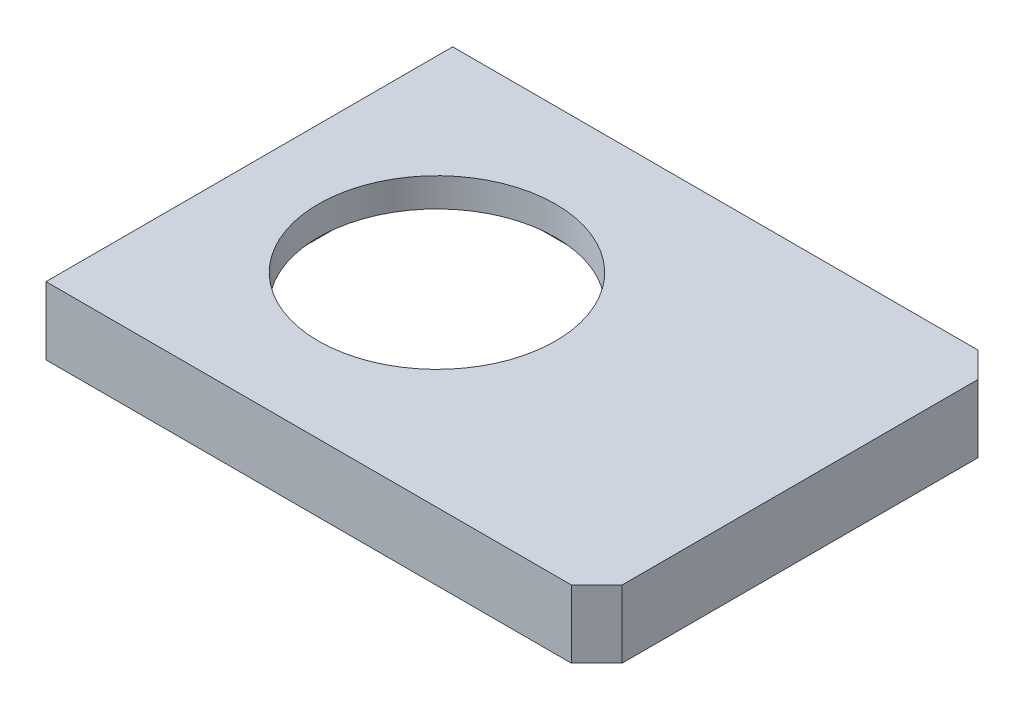
from build123d import *

# Parameters (mm, degrees)
SKETCH_1_W          = 325
SKETCH_1_H          = 240
EXTRUDE_1_DEPTH     = 40
SKETCH_2_W          = 185
SKETCH_2_H          = 185
CUT_EXTRUDE_1_DEPTH = 23
SKETCH_3_R          = 70
CUT_EXTRUDE_2_DEPTH = 204.310722787
FILLET_1_R          = 5
CHAMFER_1_SIZE      = 15


with BuildPart() as part:
    # 草图1 → 凸台-拉伸1 (new body)
    with BuildSketch(Plane(origin=(0, 0, 0), x_dir=(1, 0, 0), z_dir=(0, 1, 0))):
        Rectangle(SKETCH_1_W, SKETCH_1_H)
    extrude(amount=EXTRUDE_1_DEPTH)

    # 草图2 → 切除-拉伸1 (cut)
    with BuildSketch(Plane.XZ):
        with Locations((-51.793832524, 0)):
            Rectangle(SKETCH_2_W, SKETCH_2_H)
    extrude(amount=-CUT_EXTRUDE_1_DEPTH, mode=Mode.SUBTRACT)

    # 草图3 → 切除-拉伸2 (cut, through all)
    with BuildSketch(Plane.XZ.offset(-23)):
        with Locations(Location((-51.793832524, 0, 0), (0, 0, 270))):
            Circle(SKETCH_3_R)
    extrude(amount=-CUT_EXTRUDE_2_DEPTH, mode=Mode.SUBTRACT)

    # 圆角1
    fillet_1_edges = [part.edges().sort_by_distance(p)[0] for p in [
        (-144.293832524, 11.5, -92.5),
        (-144.293832524, 11.5, 92.5),
        (40.706167476, 11.5, 92.5),
        (40.706167476, 11.5, -92.5),
    ]]
    fillet(fillet_1_edges, radius=FILLET_1_R)

    # 倒角1
    chamfer_1_edges = [part.edges().sort_by_distance(p)[0] for p in [
        (162.5, 20, 120),
        (162.5, 20, -120),
    ]]
    chamfer(chamfer_1_edges, length=CHAMFER_1_SIZE)


solid = part.part
